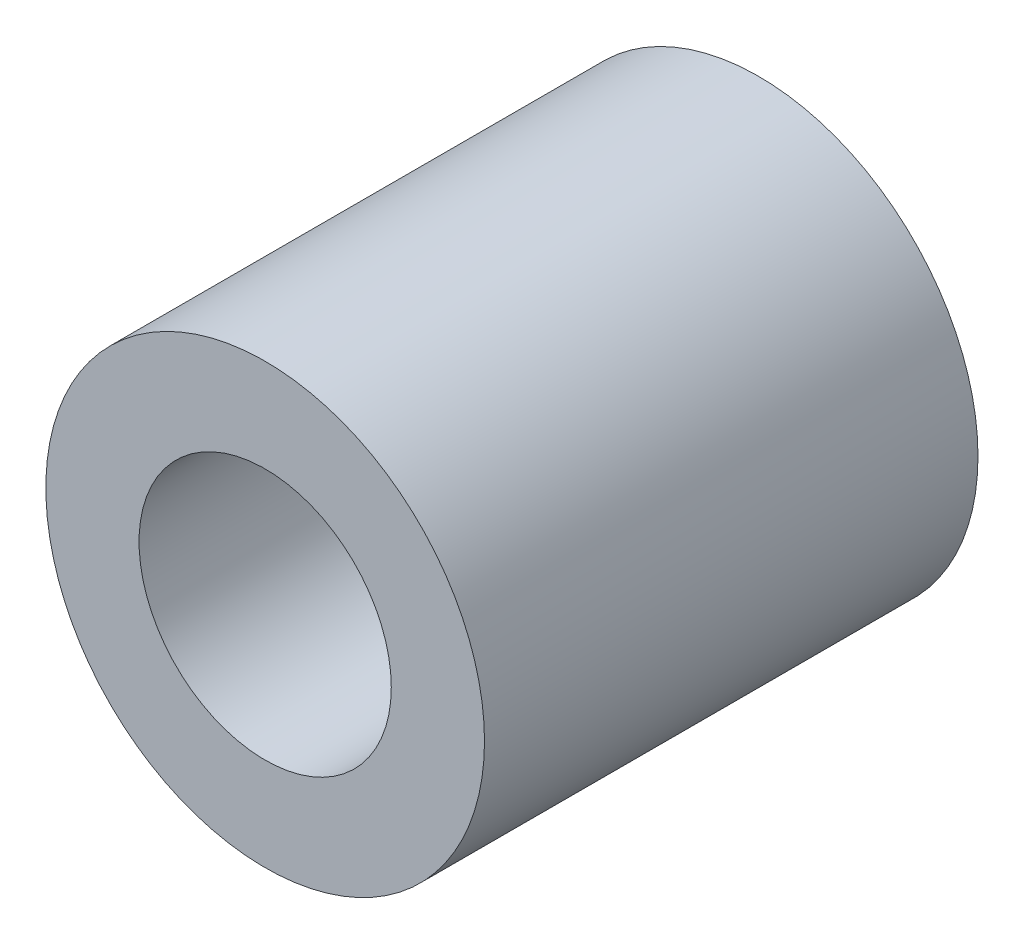
from build123d import *

# Parameters (mm, degrees)
SKETCH1_R           = 4
SKETCH1_R_2         = 2.3
BOSS_EXTRUDE1_DEPTH = 9


with BuildPart() as part:
    # Sketch1 → Boss-Extrude1 (new body)
    with BuildSketch(Plane.XY):
        Circle(SKETCH1_R)
        Circle(SKETCH1_R_2, mode=Mode.SUBTRACT)
    extrude(amount=BOSS_EXTRUDE1_DEPTH)


solid = part.part
